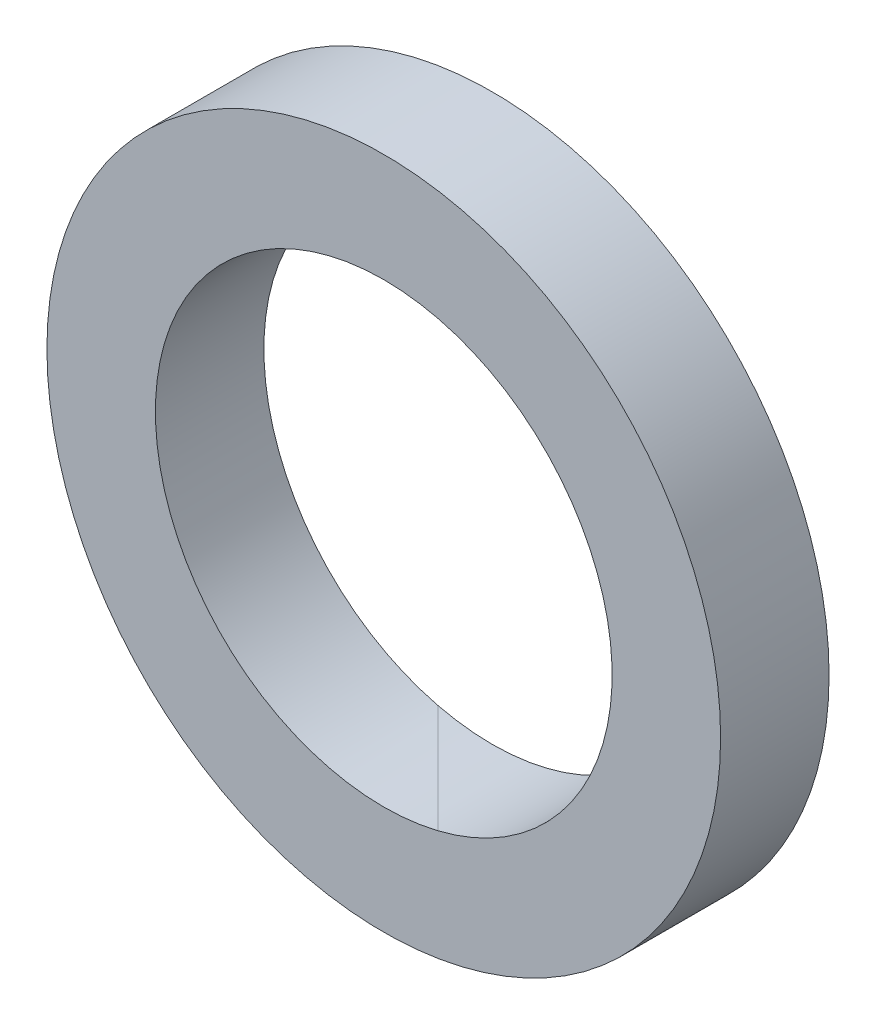
from build123d import *

# Parameters (mm, degrees)
SKETCH1_R           = 29.5
SKETCH1_R_2         = 20
BOSS_EXTRUDE1_DEPTH = 9.5


with BuildPart() as part:
    # Sketch1 → Boss-Extrude1 (new body)
    with BuildSketch(Plane.XY):
        Circle(SKETCH1_R)
        Circle(SKETCH1_R_2, mode=Mode.SUBTRACT)
    extrude(amount=BOSS_EXTRUDE1_DEPTH)


solid = part.part
